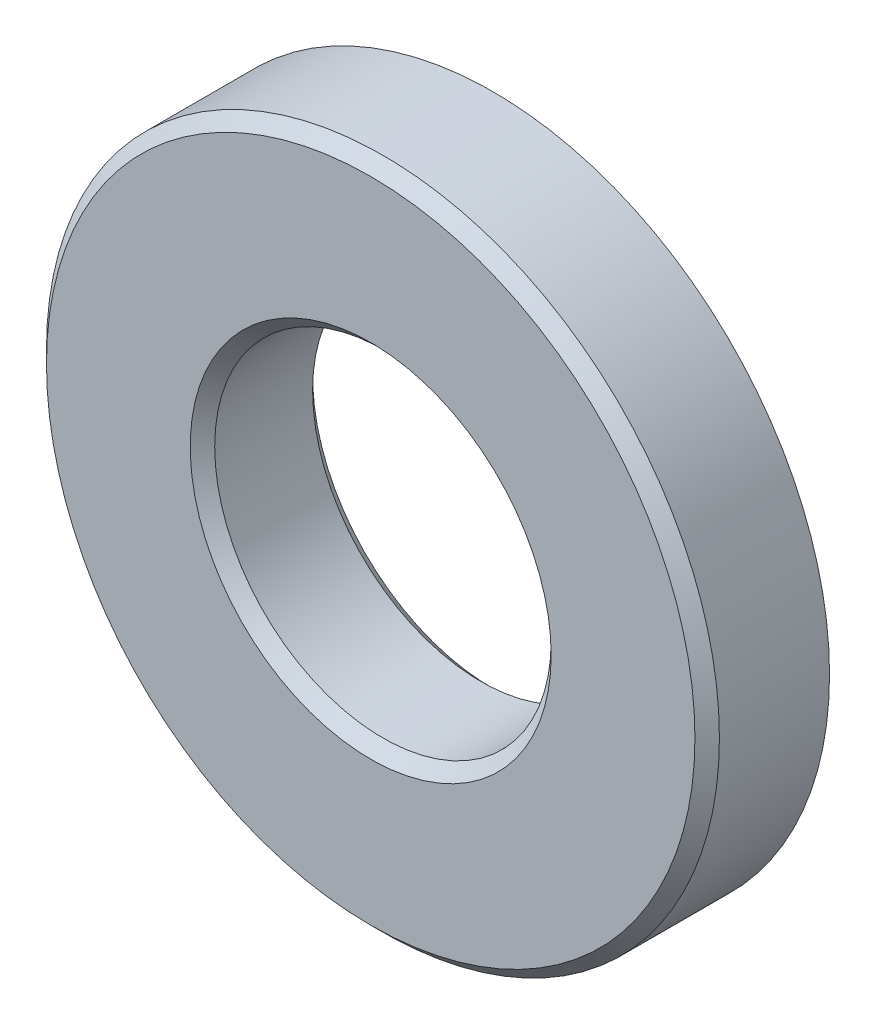
SolidWorks part; units mm, degrees
ref_plane "Front Plane" through (0, 0, 0) normal (0, 0, 1) x (1, 0, 0)
ref_plane "Top Plane" through (0, 0, 0) normal (0, 1, 0) x (1, 0, 0)
ref_plane "Right Plane" through (0, 0, 0) normal (1, 0, 0) x (0, 0, -1)
sketch "Sketch1" plane through (0, 0, 0) normal (0, 0, 1) x (1, 0, 0)
  circle A0 centre (0, 0) radius 27.5
  circle A1 centre (0, 0) radius 55
  dimension "D1" = 55
  dimension "D2" = 110
extrude "Boss-Extrude1" add sketch "Sketch1" along normal blind 20
chamfer "Chamfer1" distance 2 angle 45 3 edges at (27.5, 0, 0) (27.5, 0, 20) (55, 0, 20)
